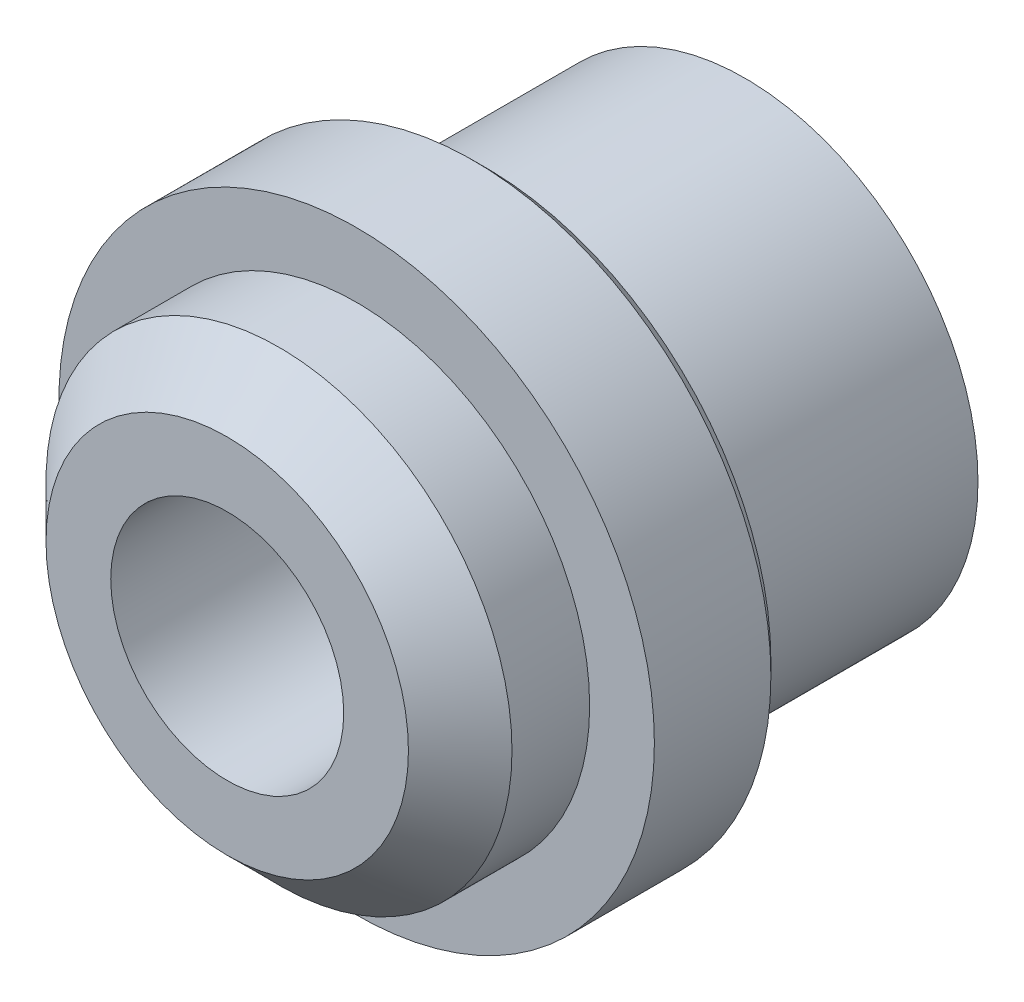
from build123d import *

# Parameters (mm, degrees)
SKETCH1_R           = 18
BOSS_EXTRUDE1_DEPTH = 20
SKETCH2_R           = 23
BOSS_EXTRUDE2_DEPTH = 10
SKETCH3_R           = 18
BOSS_EXTRUDE3_DEPTH = 10
CHAMFER1_SIZE       = 4
SKETCH4_R           = 9
CUT_EXTRUDE1_DEPTH  = 52.555795019
CHAMFER2_SIZE       = 1


with BuildPart() as part:
    # Sketch1 → Boss-Extrude1 (new body)
    with BuildSketch(Plane.XY):
        Circle(SKETCH1_R)
    extrude(amount=BOSS_EXTRUDE1_DEPTH)

    # Sketch2 → Boss-Extrude2 (add)
    with BuildSketch(Plane.XY.offset(20)):
        Circle(SKETCH2_R)
    extrude(amount=BOSS_EXTRUDE2_DEPTH)

    # Sketch3 → Boss-Extrude3 (add)
    with BuildSketch(Plane.XY.offset(30)):
        Circle(SKETCH3_R)
    extrude(amount=BOSS_EXTRUDE3_DEPTH)

    # Chamfer1
    chamfer1_edges = [part.edges().sort_by_distance(p)[0] for p in [
        (-18, 0, 40),
    ]]
    chamfer(chamfer1_edges, length=CHAMFER1_SIZE)

    # Sketch4 → Cut-Extrude1 (cut, through all)
    with BuildSketch(Plane.XY.offset(40)):
        Circle(SKETCH4_R)
    extrude(amount=-CUT_EXTRUDE1_DEPTH, mode=Mode.SUBTRACT)

    # Chamfer2
    chamfer2_edges = [part.edges().sort_by_distance(p)[0] for p in [
        (-23, 0, 20),
    ]]
    chamfer(chamfer2_edges, length=CHAMFER2_SIZE)


solid = part.part
